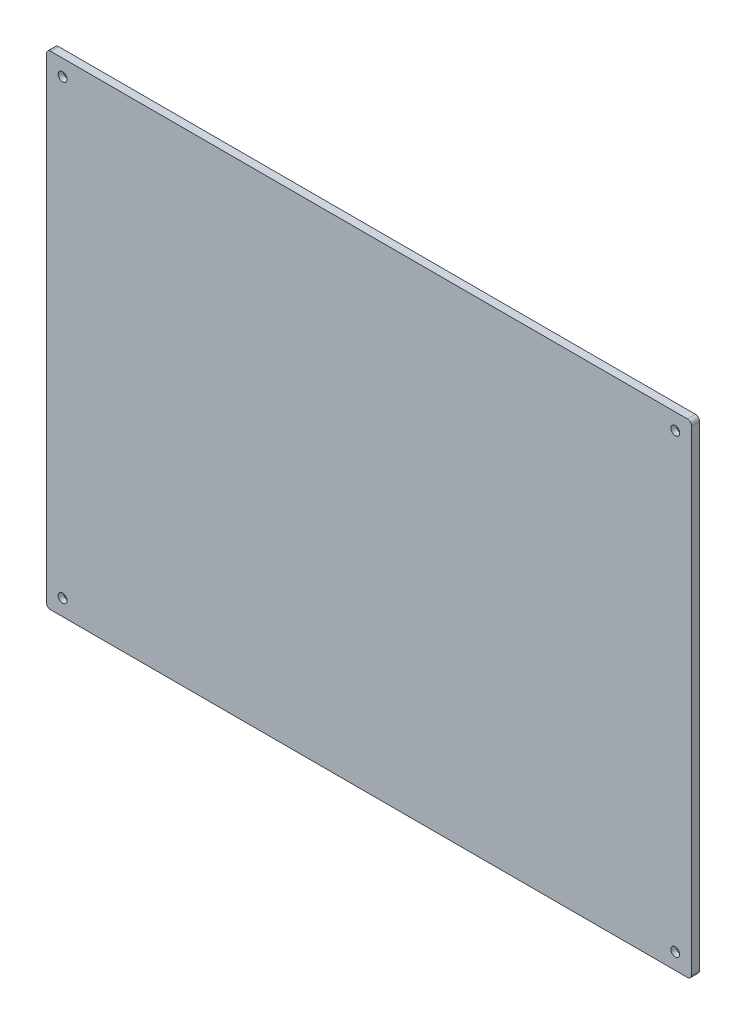
from build123d import *

# Parameters (mm, degrees)
SKETCH_1_W                   = 800
SKETCH_1_H                   = 600
EXTRUDE_1_DEPTH              = 10
HOLE_WIZARD_M6_1_D           = 6.6
HOLE_WIZARD_M6_1_CBORE_D     = 11
HOLE_WIZARD_M6_1_CBORE_DEPTH = 6.4
FILLET_1_R                   = 5


with BuildPart() as part:
    # 草图1 → 凸台-拉伸1 (new body)
    with BuildSketch(Plane.XY):
        Rectangle(SKETCH_1_W, SKETCH_1_H)
    extrude(amount=EXTRUDE_1_DEPTH)

    # M6 六角凹头螺钉的柱形沉头孔1 (through all)
    with Locations(Plane.XY.offset(10)):
        with Locations((-380, 280), (380, 280), (380, -280), (-380, -280)):
            CounterBoreHole(HOLE_WIZARD_M6_1_D / 2, HOLE_WIZARD_M6_1_CBORE_D / 2, HOLE_WIZARD_M6_1_CBORE_DEPTH)

    # 圆角1
    fillet_1_edges = [part.edges().sort_by_distance(p)[0] for p in [
        (400, -300, 5),
        (-400, -300, 5),
        (-400, 300, 5),
        (400, 300, 5),
    ]]
    fillet(fillet_1_edges, radius=FILLET_1_R)


solid = part.part
